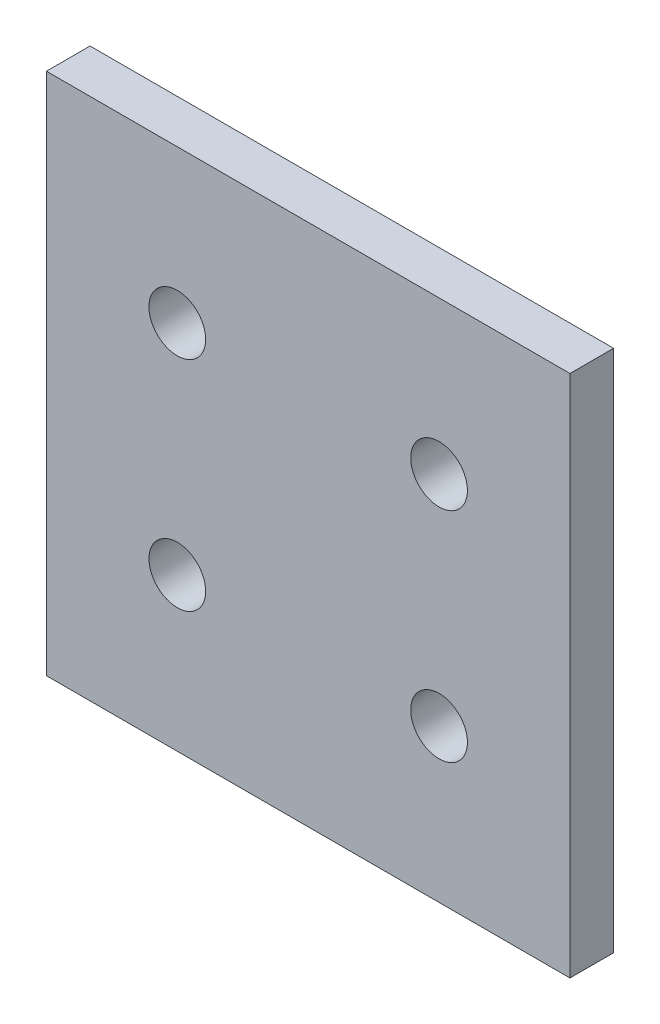
SolidWorks part; units mm, degrees
ref_plane "前视基准面" through (0, 0, 0) normal (0, 0, 1) x (1, 0, 0)
ref_plane "上视基准面" through (0, 0, 0) normal (0, 1, 0) x (1, 0, 0)
ref_plane "右视基准面" through (0, 0, 0) normal (1, 0, 0) x (0, 0, -1)
sketch "草图1" plane through (0, 0, 0) normal (0, 0, 1) x (1, 0, 0)
  line L0 (0, 0) -> (0, 120)
  line L1 (0, 120) -> (120, 120)
  line L2 (120, 120) -> (120, 0)
  line L3 (120, 0) -> (0, 0)
  line L4 (-324.875, 163.5173) -> (-264.875, 163.5173)
  line L5 (-264.875, 163.5173) -> (-264.875, 113.5173)
  line L6 (-264.875, 113.5173) -> (-324.875, 113.5173)
  line L7 (-324.875, 113.5173) -> (-324.875, 163.5173)
  line L9 (-324.875, 163.5173) -> (-264.875, 113.5173)
  line L10 (30, 41.5) -> (30, 78.5)
  line L11 (83.5, 35) -> (36.5, 35)
  line L12 (90, 78.5) -> (90, 41.5)
  line L14 (36.5, 85) -> (83.5, 85)
  line L16 (91.3568, 28.6432) -> (120, 0)
  circle A0 centre (-324.875, 163.5173) radius 6.5
  circle A1 centre (-264.875, 163.5173) radius 6.5
  circle A2 centre (-264.875, 113.5173) radius 6.5
  circle A3 centre (-324.875, 113.5173) radius 6.5
  circle A4 centre (90, 35) radius 6.5
  circle A5 centre (30, 85) radius 6.5
  circle A6 centre (90, 85) radius 6.5
  circle A7 centre (30, 35) radius 6.5
extrude "凸台-拉伸1" add sketch "草图1" along normal blind 10
